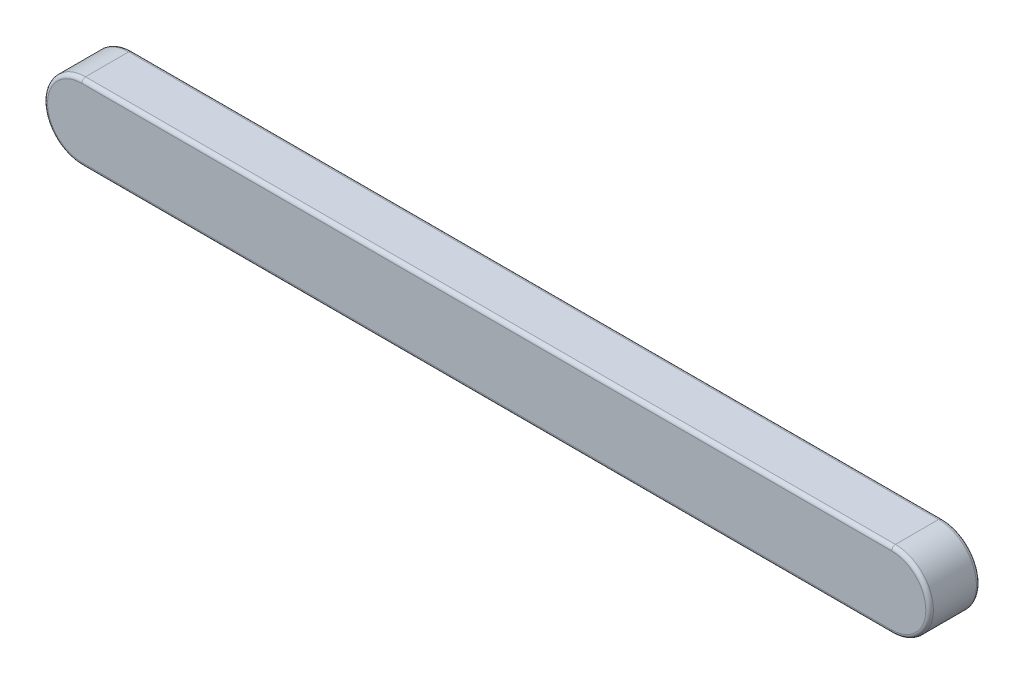
SolidWorks part; units mm, degrees
material "45"
ref_plane "基准面1" through (0, 0, 0) normal (0, 0, 1) x (1, 0, 0)
ref_plane "基准面2" through (0, 0, 0) normal (0, 1, 0) x (1, 0, 0)
ref_plane "基准面3" through (0, 0, 0) normal (1, 0, 0) x (0, 0, -1)
sketch "尺寸草图" plane through (0, 0, 0) normal (0, 0, 1) x (1, 0, 0)
  line L0 (-70, 0) -> (70, 0) construction
  point P3 (-8, 0)
  point P4 (-0.6, 0)
  point P5 (0, 0)
  point P8 (-12, 0)
  point P11 (0, 0)
sketch "草图1" plane through (0, 0, 0) normal (0, 0, 1) x (1, 0, 0)
  line L0 (-28.0599, 0) -> (30.562, 0) construction
  line L1 (-64, 6) -> (64, 6)
  line L2 (-64, -6) -> (64, -6)
  line L3 (0, 2.9108) -> (0, -2.1805) construction
  arc A0 (-64, 6) -> (-64, -6) centre (-64, 0) ccw
  arc A1 (64, 6) -> (64, -6) centre (64, 0) cw
extrude "基体-拉伸" add sketch "草图1" along normal blind 8
fillet "圆角1" radius 0.6 8 edges at (70, 0, 8) (0, 6, 8) (-70, 0, 8) (0, 6, 0) (70, 0, 0) (0, -6, 0) (-70, 0, 0) (0, -6, 8)
equation "\"D3@草图1\" = \"L@尺寸草图\""
equation "\"D1@草图1\" = \"b@尺寸草图\" / 2"
equation "\"D1@圆角1\" = \"r@尺寸草图\""
equation "\"D1@基体-拉伸\" = \"h@尺寸草图\""
